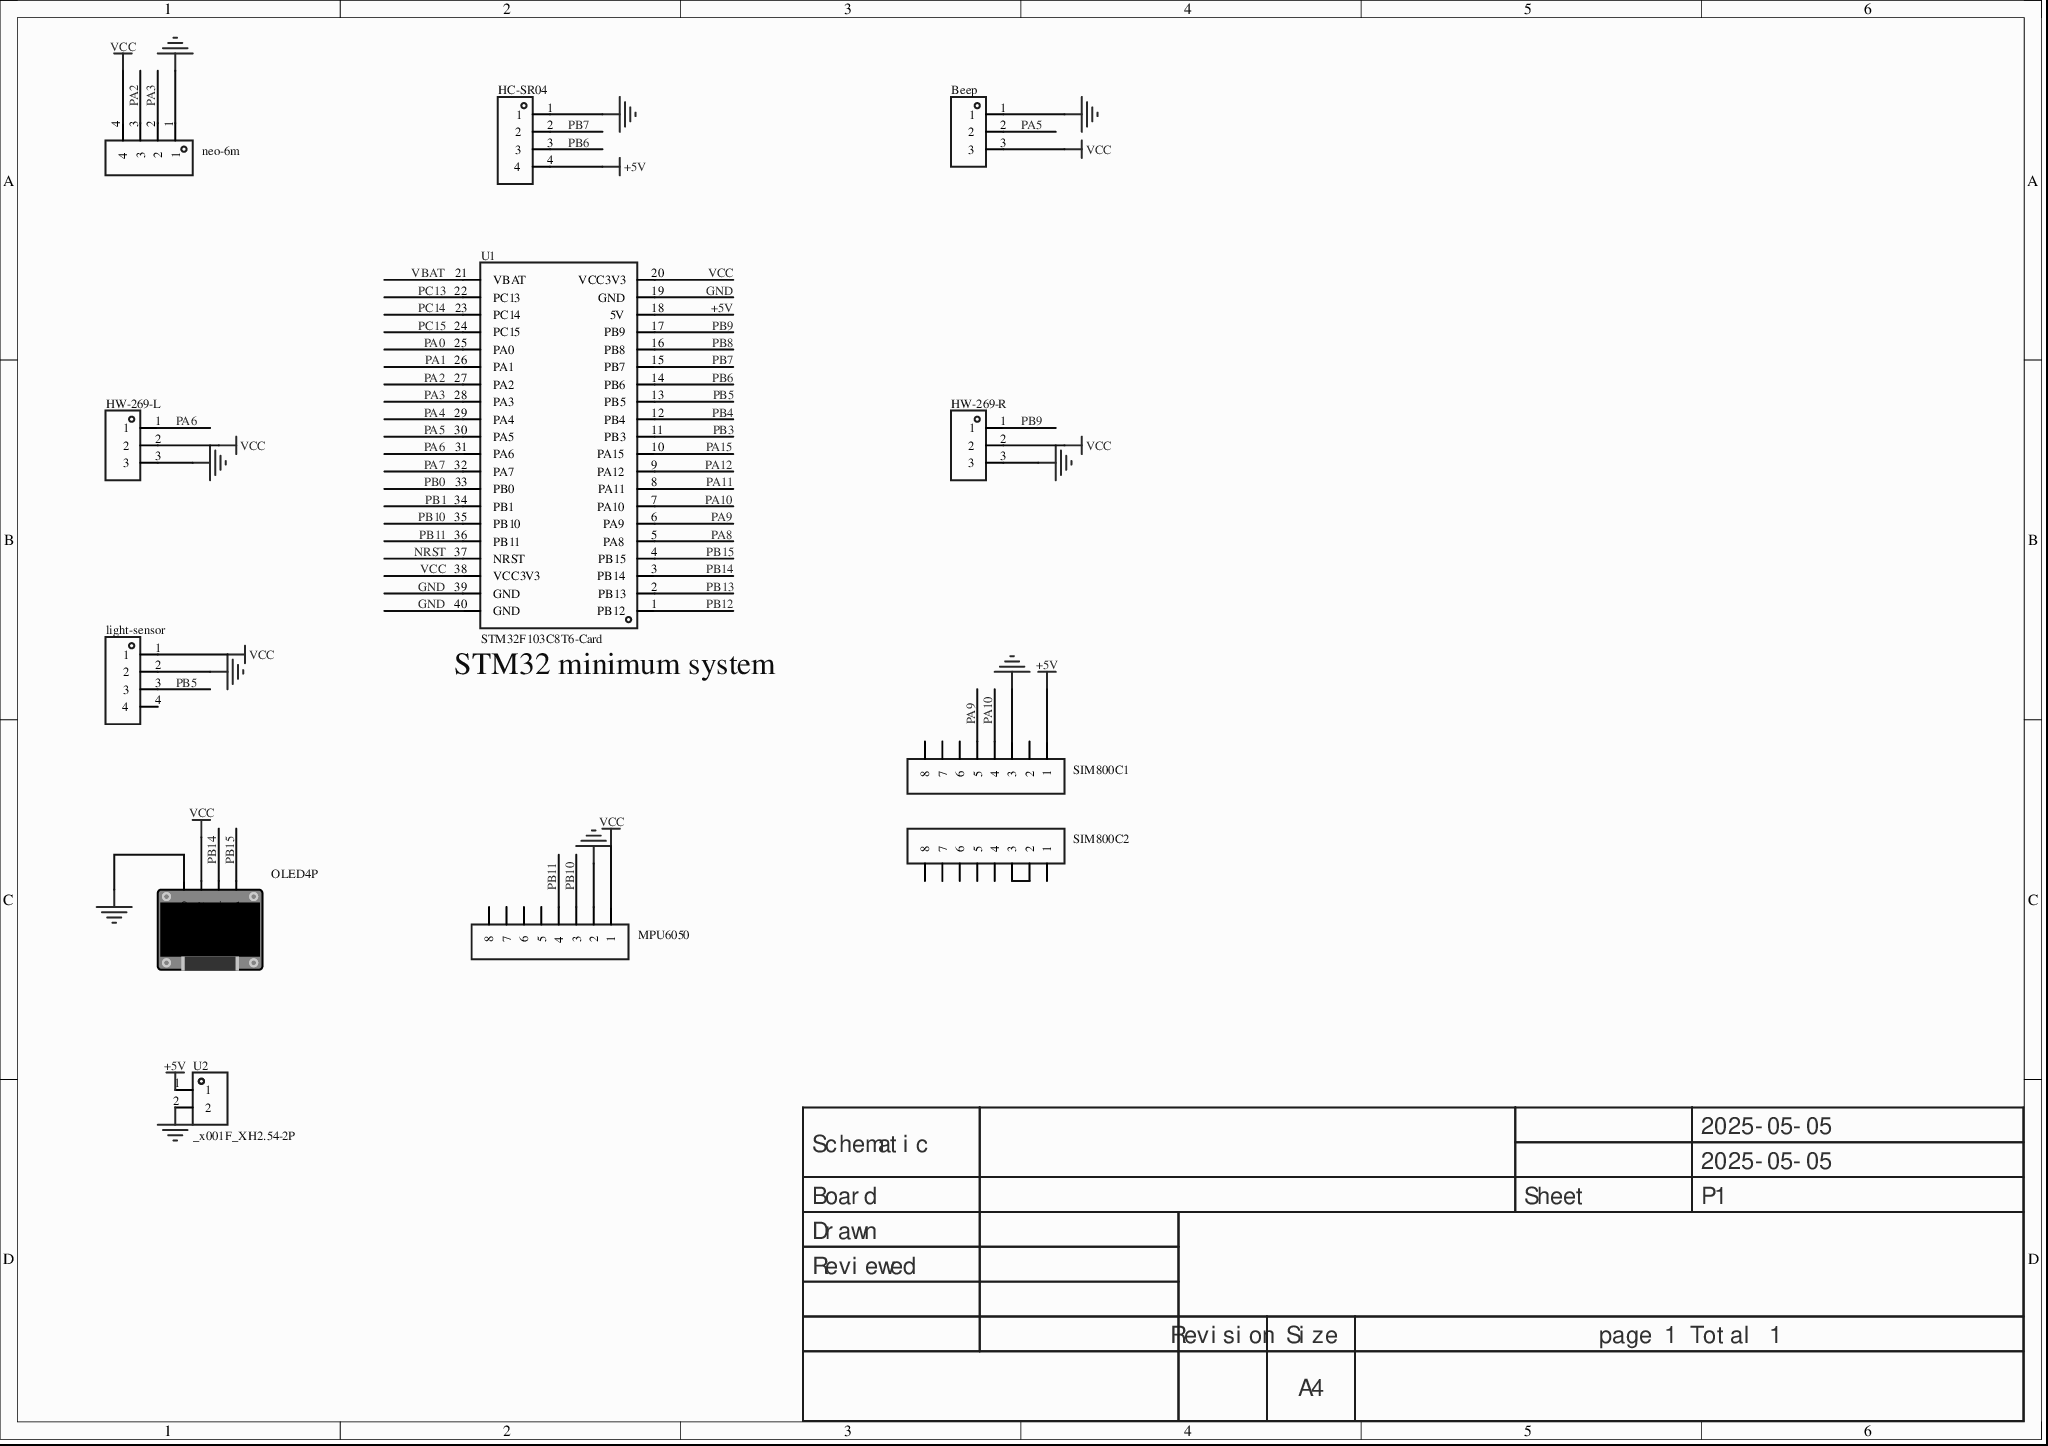
[diagram p0: MISC51587-3.schdoc]
# Altium project MISC51587-2.PrjPcb
1 sheet, 12 parts. Net scope: global (net labels, ports and power ports of the same name join across sheets).
Board file: MISC51587.pcbdoc

## Sheet MISC51587-3.schdoc
size 297 x 209 mm; Version: V1.0; @Project Name: MISC51587; @Page Count: 1; @Update Date: 2025-05-05; @Create Date: 2025-05-05; @Schematic Name: MISC51587; @Page No: 1; @Create Time: 19:21:47; @Update Time: 20:34:39; @Board Name: MISC51587

### Parts
Beep  (no value)  [HDR-TH_3P-P2.54-V-F]
HC-SR04  (no value)  [HDR-TH_4P-P2.54-V-F]
HW-269-L  (no value)  [HDR-TH_3P-P2.54-V-F]
HW-269-R  (no value)  [HDR-TH_3P-P2.54-V-F]
light-sensor  (no value)  [HDR-TH_4P-P2.54-V-F]
MPU6050  (no value)  [HDR-TH_8P-P2.54-V-F-1]
neo-6m  (no value)  [HDR-TH_4P-P2.54-V-F]
OLED4P  (no value)  [0.96OLED_4P]
SIM800C1  (no value)  [HDR-TH_8P-P2.54-V-F-1]
SIM800C2  (no value)  [HDR-TH_8P-P2.54-V-F-1]
U1  STM32F103C8T6-Card  [CONN-TH_L53.3-W22.9_STM32F103C8T6-CARD]
U2  _x001F_XH2.54-2P  [CONN-TH_2P-P2.54-V]

### Nets
+5V: HC-SR04.4 SIM800C1.1 U1.18(5V) U2.1
GND: Beep.1 HC-SR04.1 HW-269-L.3 HW-269-R.3 light-sensor.2 MPU6050.2 neo-6m.1 OLED4P.1(GND) SIM800C1.3 U1.19(GND) U1.39(GND) U1.40(GND) U2.2
VCC: Beep.3 HW-269-L.2 HW-269-R.2 light-sensor.1 MPU6050.1 neo-6m.4 OLED4P.2(VCC) U1.20(VCC3V3) U1.38(VCC3V3)
NRST: U1.37(NRST)
PA0: U1.25(PA0)
PA1: U1.26(PA1)
PA2: neo-6m.3 U1.27(PA2)
PA3: neo-6m.2 U1.28(PA3)
PA4: U1.29(PA4)
PA5: Beep.2 U1.30(PA5)
PA6: HW-269-L.1 U1.31(PA6)
PA7: U1.32(PA7)
PA8: U1.5(PA8)
PA9: SIM800C1.5 U1.6(PA9)
PA10: SIM800C1.4 U1.7(PA10)
PA11: U1.8(PA11)
PA12: U1.9(PA12)
PA15: U1.10(PA15)
PB0: U1.33(PB0)
PB1: U1.34(PB1)
PB3: U1.11(PB3)
PB4: U1.12(PB4)
PB5: light-sensor.3 U1.13(PB5)
PB6: HC-SR04.3 U1.14(PB6)
PB7: HC-SR04.2 U1.15(PB7)
PB8: U1.16(PB8)
PB9: HW-269-R.1 U1.17(PB9)
PB10: MPU6050.3 U1.35(PB10)
PB11: MPU6050.4 U1.36(PB11)
PB12: U1.1(PB12)
PB13: U1.2(PB13)
PB14: OLED4P.3(SCL) U1.3(PB14)
PB15: OLED4P.4(SDA) U1.4(PB15)
PC13: U1.22(PC13)
PC14: U1.23(PC14)
PC15: U1.24(PC15)
VBAT: U1.21(VBAT)
NetSIM800C2_2: SIM800C2.2 SIM800C2.3

Not connected (* = marked no-connect by the designer): light-sensor 4*; MPU6050 5* 6* 7* 8*; SIM800C1 2* 6* 7* 8; SIM800C2 1 4* 5* 6* 7* 8*

### Notes on the sheet
- (near U1) STM32 minimum system
- 2025-05-05
- Schematic
- Board
- Sheet
- P1
- Drawn
- Reviewed
- Revision
- Size
- A4
- page 1 Total 1

### Library data of the parts
Beep HW-269-L HW-269-R = HDR-F_2.54_1x3P: Symbol: PM254V-11-03-H85; ConvertToPcb: yes; ModelId: f3b3cc5aae9641bf9e56fc160cef875b; ModelName: HDR2.54-F-LI-1X3P; ModelTransform: 299.9994,100,0,0,0,0,0,0,-118.11; Device: HDR-F_2.54_1x3P; AddInBom: yes; SupplierPart: C541850; Supplier Footprint: 插件; FootprintName: HDR-TH_3P-P2.54-V-F
HC-SR04 light-sensor neo-6m = HDR-F_2.54_1x4P: ConvertToPcb: yes; SymbolName: 2.54-1*4P female; ModelId: d187812051054f85879fcaa51a310d8e; ModelTransform: 419.6842,98.464,0,0,0,0,0,0,-118.11; Device: HDR-F_2.54_1x4P; AddInBom: yes; SupplierPart: C2718488; Supplier Footprint: 插件; FootprintName: HDR-TH_4P-P2.54-V-F; ModelName: HDR-TH_4P-P2.54-V-F
MPU6050 SIM800C1 SIM800C2 = HDR-F_2.54_1x8P: Symbol: Header-Female-2.54_1x8; AddInBom: yes; ModelId: 0f7e4d9227ef4fa08d5469c22cc70cdb; ModelName: HDR-F-2.54_1x8; ModelTransform: 799.99844,100,0,0,0,0,0,0,-118.11; Device: HDR-F_2.54_1x8P; ConvertToPcb: yes; FootprintName: HDR-TH_8P-P2.54-V-F-1; SupplierPart: C27438; Supplier Footprint: 插件
OLED4P = 0.96OLED模块_4P: Device: 0.96OLED module_4P; ConvertToPcb: yes; ModelId: 79c000fdb68d45a296c2e9bedf4f9055; ModelTransform: 1393.69792,1318.895,0,0,0,0,0,-560.079,-137.795; AddInBom: yes; SymbolName: 0.96OLED module_4P; FootprintName: 0.96OLED_4P; Supplier Footprint: 插件; ModelName: 0.96OLED_4P
U1 = STM32F103C8T6-Card: AddInBom: yes; Symbol: STM32F103C8T6-CARD; Device: STM32F103C8T6-Card; LCSC Part Name: STM32F103C8T6-Card; SupplierPart: C9900077949; ManufacturerPart: STM32F103C8T6-Card; Supplier Footprint: 插件; Supplier: LCSC; ConvertToPcb: yes; FootprintName: CONN-TH_L53.3-W22.9_STM32F103C8T6-CARD
U2 = _x001F_XH2.54-2P: AddInBom: yes; ModelId: 4b619f877c224111ac90f050b36c3583; ModelTransform: 295.275,224.409,0,180,0,0,0,17.717,-118.11; Symbol: _X001F_XH2.54-2P; Device: _x001F_XH2.54-2P; LCSC Part Name: _x001F_XH2.54-2P; SupplierPart: C9900016027; ManufacturerPart: _x001F_XH2.54-2P; Supplier Footprint: XH2.54-2P直插; JLCPCB Part Class: Extended library; Supplier: LCSC; ConvertToPcb: yes; FootprintName: CONN-TH_2P-P2.54-V; ModelName: CONN-TH_2P-P2.54-V